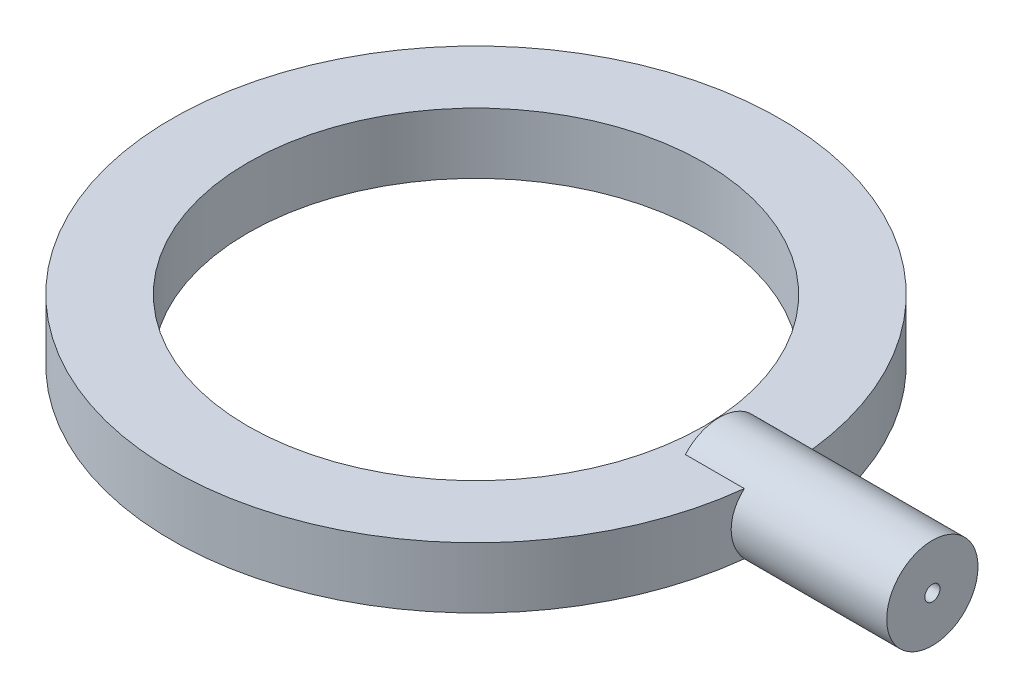
SolidWorks part; units mm, degrees
ref_plane "Front Plane" through (0, 0, 0) normal (0, 0, 1) x (1, 0, 0)
ref_plane "Top Plane" through (0, 0, 0) normal (0, 1, 0) x (1, 0, 0)
ref_plane "Right Plane" through (0, 0, 0) normal (1, 0, 0) x (0, 0, -1)
sketch "Sketch1" plane through (0, 0, 0) normal (0, 1, 0) x (1, 0, 0)
  circle A0 centre (0, 0) radius 100
  circle A1 centre (0, 0) radius 75
  dimension "D1" = 200
  dimension "D2" = 150
extrude "Boss-Extrude1" add sketch "Sketch1" along normal blind 20
sketch "Sketch2" plane through (0, 0, 0) normal (1, 0, 0) x (0, 0, -1)
  circle A0 centre (0, 10) radius 15
  dimension "D1" = 30
  dimension "D2" = 10
extrude "Boss-Extrude2" add sketch "Sketch2" along normal blind 70 from offset 80
hole_wizard "M6 Tapped Hole1" positions "Sketch3" profile "Sketch4" tap size "M6" standard "GB"
sketch "Sketch3" plane through (150, 0, 0) normal (1, 0, 0) x (0, 0, -1)
  point P0 (0, 10)
sketch "Sketch4" plane through (150, 10, 0) normal (0, 1, 0) x (0, 0, -1)
  line L0 (0, 0) -> (0, 18.5022)
  line L1 (0, 18.5022) -> (2.5, 17)
  line L2 (2.5, 17) -> (2.5, 0)
  line L5 (2.5, 0) -> (0, 0)
  line L10 (0, 18.5022) -> (-2.5, 17) construction
  line L11 (0, -6.35) -> (0, 107.95) construction
  dimension "螺纹孔钻头直径" = 5
  dimension "螺纹孔钻头深度" = 17
  dimension "导头角度" = 118
cosmetic thread "Hole thread 1" parameters "D1"=12, "D2"=6
